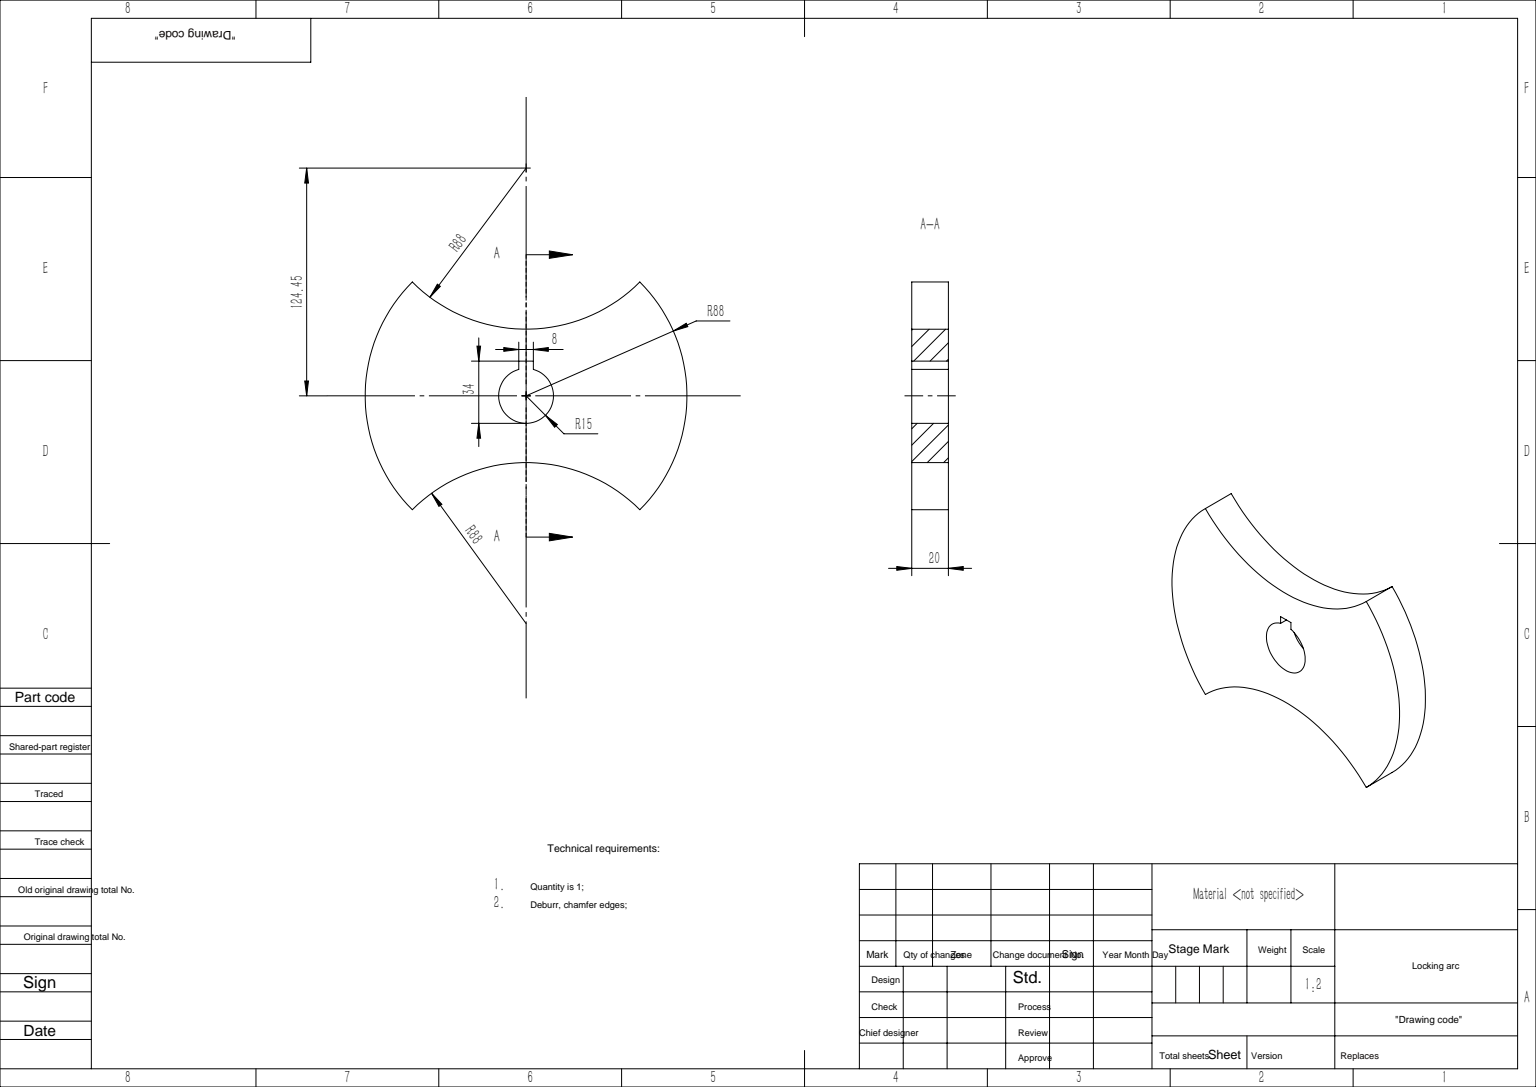
SolidWorks part; units mm, degrees
ref_plane "前视基准面" through (0, 0, 0) normal (0, 0, 1) x (1, 0, 0)
ref_plane "上视基准面" through (0, 0, 0) normal (0, 1, 0) x (1, 0, 0)
ref_plane "右视基准面" through (0, 0, 0) normal (1, 0, 0) x (0, 0, -1)
sketch "草图1" plane through (0, 0, 0) normal (0, 0, 1) x (1, 0, 0)
  line L0 (-150, 0) -> (150, 0) construction
  line L1 (0, 150) -> (0, -150) construction
  line L2 (0, 0) -> (-62.2254, -62.2254) construction
  line L3 (0, 0) -> (62.2254, -62.2254) construction
  arc A0 (-62.2254, 62.2254) -> (-62.2254, -62.2254) centre (0, 0) ccw
  arc A1 (-62.2254, -62.2254) -> (62.2254, -62.2254) centre (0, -124.4508) cw
  arc A2 (-62.2254, 62.2254) -> (62.2254, 62.2254) centre (0, 124.4508) ccw
  arc A3 (62.2254, -62.2254) -> (62.2254, 62.2254) centre (0, 0) ccw
  dimension "D1" = 176
  dimension "D4" = 90
  dimension "D6" = 88
  dimension "D2" = 300
  dimension "D3" = 300
  dimension "D5" = 45
extrude "凸台-拉伸1" add sketch "草图1" along normal blind 20
sketch "草图2" plane through (0, 0, 20) normal (0, 0, 1) x (1, 0, 0)
  line L0 (0, 0) -> (0, 59.4184) construction
  line L1 (-4, 19) -> (4, 19)
  line L2 (-4, 19) -> (-4, 14.4568)
  line L4 (4, 19) -> (4, 14.4568)
  arc A0 (-4, 14.4568) -> (4, 14.4568) centre (0, 0) ccw
  dimension "D1" = 30
  dimension "D2" = 8
  dimension "D3" = 19
extrude "切除-拉伸1" cut sketch "草图2" against normal through all
